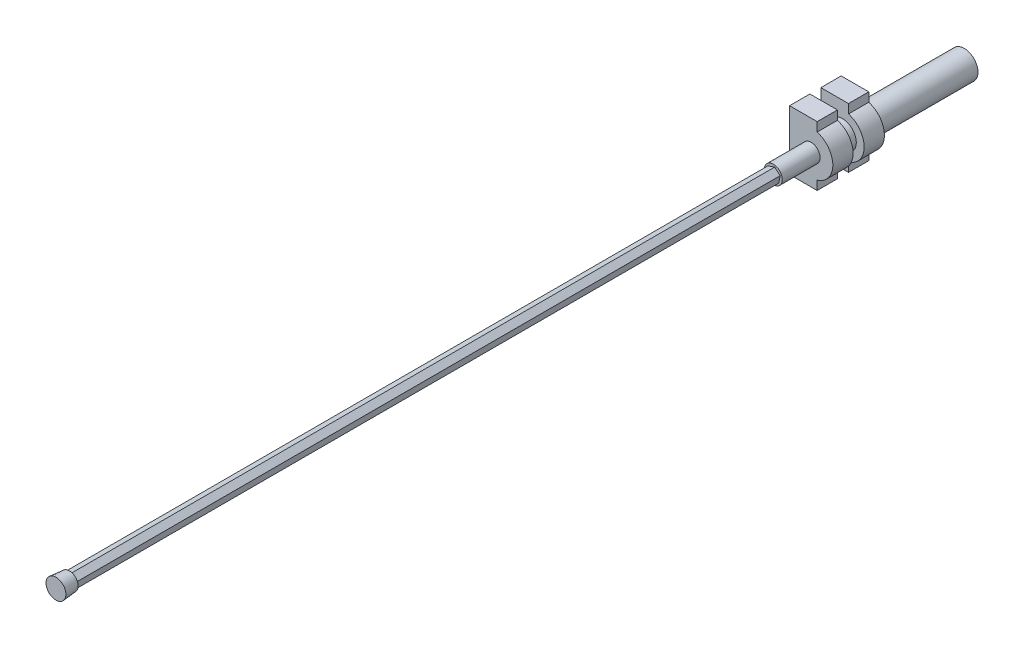
SolidWorks part; units mm, degrees
ref_plane "Front Plane" through (0, 0, 0) normal (0, 0, 1) x (1, 0, 0)
ref_plane "Top Plane" through (0, 0, 0) normal (0, 1, 0) x (1, 0, 0)
ref_plane "Right Plane" through (0, 0, 0) normal (1, 0, 0) x (0, 0, -1)
sketch "Sketch1" plane through (0, 0, 0) normal (0, 0, 1) x (1, 0, 0)
  circle A0 centre (0, 0) radius 46.2
  dimension "D1" = 92.4
extrude "Boss-Extrude1" add sketch "Sketch1" along normal blind 445
sketch "Sketch2" plane through (0, 0, 445) normal (0, 0, 1) x (1, 0, 0)
  circle A0 centre (0, 0) radius 30
  dimension "D1" = 60
extrude "Boss-Extrude2" add sketch "Sketch2" along normal blind 195
sketch "Sketch3" plane through (0, 0, 640) normal (0, 0, 1) x (1, 0, 0)
  line L1 (18.3419, -15.8611) -> (22.9071, 7.954)
  line L2 (22.9071, 7.954) -> (4.5652, 23.8151)
  line L3 (4.5652, 23.8151) -> (-18.3419, 15.8611)
  line L4 (-18.3419, 15.8611) -> (-22.9071, -7.954)
  line L5 (-22.9071, -7.954) -> (-4.5652, -23.8151)
  line L6 (-4.5652, -23.8151) -> (18.3419, -15.8611)
  circle A0 centre (0, 0) radius 21 construction
  dimension "D1" = 42
extrude "Boss-Extrude3" add sketch "Sketch3" along normal blind 2360
sketch "Sketch4" plane through (0, 0, 0) normal (0, 1, 0) x (1, 0, 0)
  line L1 (4.5652, -3000) -> (-18.3419, -3000) construction
  line L2 (0, 0) -> (0, -5371.757) construction
  line L4 (29.4, -3000) -> (0, -3000)
  line L5 (29.4, -3000) -> (33.3, -3045)
  line L6 (33.3, -3045) -> (0, -3045)
  line L7 (0, -3000) -> (0, -3045)
  dimension "D1" = 29.4
  dimension "D2" = 33.3
  dimension "D3" = 45
revolve "Revolve1" add sketch "Sketch4" angle 360 about L2
sketch "Sketch5" plane through (0, 0, 445) normal (0, 0, 1) x (1, 0, 0)
  line L0 (0, 0) -> (-215.4684, 0) construction
  line L1 (0, 0) -> (0, 267.7695) construction
  line L2 (0, 100) -> (-72.5, 100)
  line L3 (-72.5, 100) -> (-72.5, -100)
  line L4 (0, 100) -> (20, 100)
  line L5 (20, 100) -> (20, 69.6868)
  line L6 (0, -100) -> (-72.5, -100)
  line L7 (0, -100) -> (20, -100)
  line L8 (20, -100) -> (20, -69.6868)
  arc A0 (20, -69.6868) -> (20, 69.6868) centre (0, 0) ccw
  dimension "D1" = 145
  dimension "D2" = 100
  dimension "D3" = 20
extrude "Boss-Extrude4" add sketch "Sketch5" along normal blind 68
ref_plane "Plane1" through (0, 0, 340) normal (0, 0, 1) x (1, 0, 0)
sketch "Sketch6" plane through (0, 0, 340) normal (0, 0, 1) x (1, 0, 0)
  line L5 (20, 100) -> (-72.5, 100)
  line L6 (20, 69.6868) -> (20, 100)
  line L7 (20, -100) -> (20, -69.6868)
  line L8 (-72.5, -100) -> (20, -100)
  line L9 (-72.5, 100) -> (-72.5, -100)
  line L10 (20, 100) -> (-72.5, 100)
  line L11 (20, 69.6868) -> (20, 100)
  line L12 (20, -100) -> (20, -69.6868)
  line L13 (-72.5, -100) -> (20, -100)
  line L14 (-72.5, 100) -> (-72.5, -100)
  arc A1 (20, -69.6868) -> (20, 69.6868) centre (0, 0) ccw
  arc A2 (20, -69.6868) -> (20, 69.6868) centre (0, 0) ccw
  dimension "D1" = 0
extrude "Boss-Extrude5" add sketch "Sketch6" along normal blind 68
